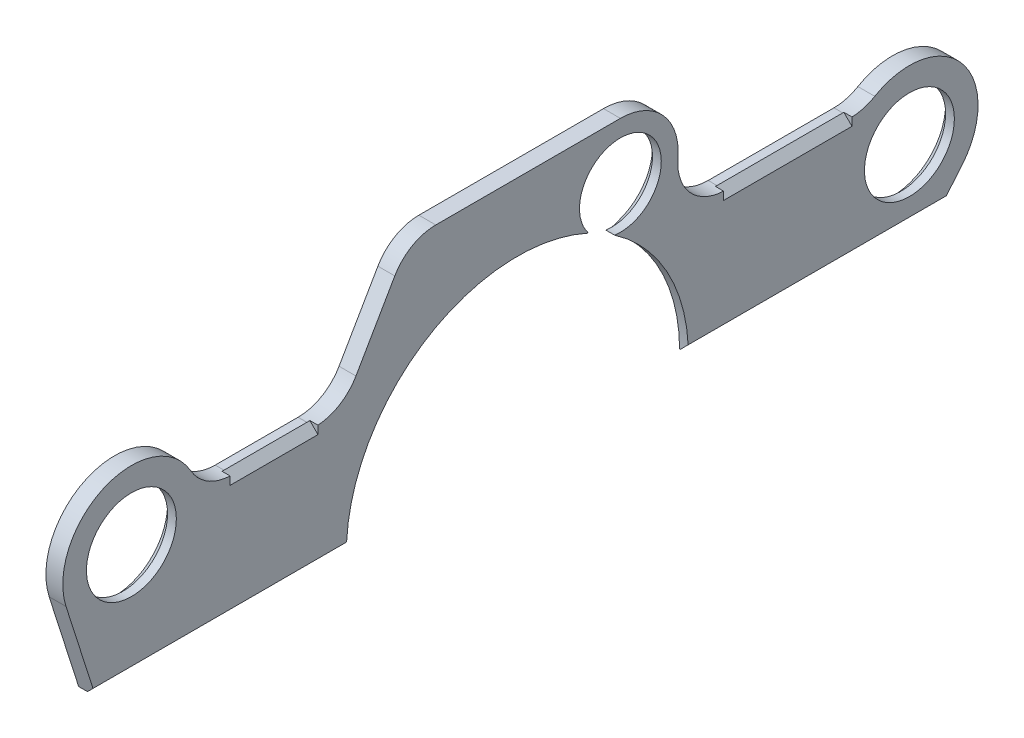
SolidWorks part; units mm, degrees
material "Q345B"
ref_plane "Front Plane" through (0, 0, 0) normal (0, 0, 1) x (1, 0, 0)
ref_plane "Top Plane" through (0, 0, 0) normal (0, 1, 0) x (1, 0, 0)
ref_plane "Right Plane" through (0, 0, 0) normal (1, 0, 0) x (0, 0, -1)
sketch "Sketch1" plane through (0, 0, 0) normal (1, 0, 0) x (0, 0, -1)
  line L0 (-1867.4529, 0) -> (418.1387, 0) construction
  line L1 (0, 339.4389) -> (0, -315.5279) construction
  line L2 (-161.1391, 353.5) -> (152.4, 353.5)
  line L3 (-161.1391, 353.5) -> (-259, 184)
  line L4 (-470.6145, 184) -> (-259, 184)
  line L6 (657.7535, 40.7571) -> (624.5612, 1.2)
  line L7 (307.2685, 184) -> (515.0519, 184)
  line L9 (-624, 1.2) -> (-667.6968, 138.1459)
  line L10 (624.5612, 1.2) -> (252.9972, 1.2)
  line L12 (-624, 1.2) -> (-252.9972, 1.2)
  arc A0 (237.5528, 260.3023) -> (307.2685, 184) centre (307.2685, 254) ccw
  arc A1 (252.9972, 1.2) -> (-252.9972, 1.2) centre (0, 0) ccw
  arc A2 (657.7535, 40.7571) -> (515.0519, 184) centre (580, 106) ccw
  arc A3 (-470.6145, 184) -> (-667.6968, 138.1459) centre (-571, 169) ccw
  arc A5 (237.5528, 260.3023) -> (152.4, 353.5) centre (152.4, 268) ccw
  dimension "D1" = 253
  dimension "D8" = 259
  dimension "D2" = 60
  dimension "D3" = 101.5
  dimension "D14" = 85.5
  dimension "D16" = 70
  dimension "D5" = 106
  dimension "D6" = 169
  dimension "D7" = 50
  dimension "D9" = 571
  dimension "D10" = 624
  dimension "D11" = 580
  dimension "D12" = 152.4
  dimension "D13" = 268
  dimension "D15" = 184
  dimension "D17" = 1.2
extrude "Boss-Extrude1" add sketch "Sketch1" along normal mid plane 25
sketch "Sketch2" plane through (0, 0, 0) normal (1, 0, 0) x (0, 0, -1)
  line L2 (-759.6656, 0) -> (783.6604, 0) construction
  line L3 (0, -128.1309) -> (0, 556.7634) construction
  circle A0 centre (152.4, 268) radius 60.5
  circle A1 centre (-571, 169) radius 66.5
  circle A2 centre (580, 106) radius 66.5
  dimension "D3" = 121
  dimension "D4" = 133
  dimension "D1" = 152.4
  dimension "D2" = 268
extrude "Cut-Extrude1" cut sketch "Sketch2" against normal through all both and the other way through all
fillet "Fillet1" radius 70 4 edges at (0, 184, -515.0519) (0, 353.5, 161.1391) (0, 184, 259) (0, 184, 470.6145)
chamfer "Chamfer1" distance 12 angle 45 2 edges at (12.5, 1.2, -438.7792) (12.5, 1.2, 438.4986)
chamfer "Chamfer2" distance 12 angle 45 5 edges at (-12.5, 169, 504.5) (-12.5, 106, -646.5) (-12.5, 213.2137, 136.1944) (-12.5, 320.5914, -182.3064) (-12.5, 118.0184, -223.7871)
ref_plane "Plane1" through (0, 0, 360) normal (0, 0, 1) x (1, 0, 0)
ref_plane "Plane2" through (0, 0, -400) normal (0, 0, 1) x (1, 0, 0)
sketch "Sketch3" plane through (0, 0, 360) normal (0, 0, 1) x (1, 0, 0)
  line L0 (-5.5, 190) -> (12.5, 172)
  line L1 (12.5, 172) -> (12.5, 190)
  line L3 (12.5, 138.1459) -> (12.5, 270.5) construction
  line L5 (-5.5, 190) -> (12.5, 190)
  dimension "D1" = 45
  dimension "D2" = 172
  dimension "D4" = 190
extrude "Cut-Extrude2" cut sketch "Sketch3" against normal mid plane 130
sketch "Sketch4" plane through (0, 0, -400) normal (0, 0, 1) x (1, 0, 0)
  line L4 (12.5, 190) -> (-5.5, 190)
  line L5 (12.5, 190) -> (-5.5, 190)
  line L6 (-5.5, 190) -> (12.5, 172)
  line L7 (12.5, 172) -> (12.5, 190)
  line L9 (-5.5, 190) -> (12.5, 172)
  line L10 (12.5, 172) -> (12.5, 190)
  dimension "D1" = 0
extrude "Cut-Extrude3" cut sketch "Sketch4" against normal mid plane 190
